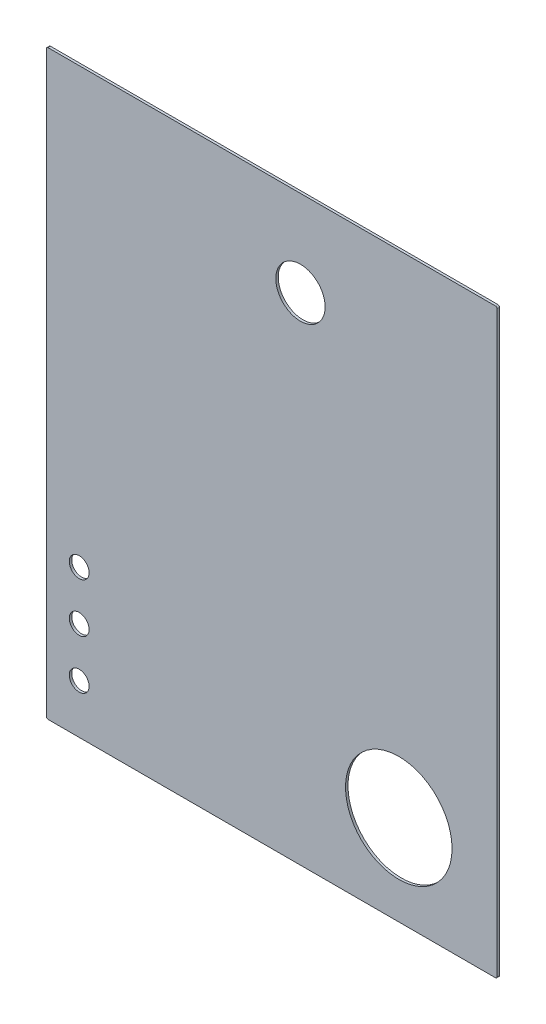
from build123d import *

# Parameters (mm, degrees)
SKETCH1_R           = 12.1
SKETCH1_R_2         = 65
SKETCH1_R_3         = 30.1
BOSS_EXTRUDE1_DEPTH = 3


with BuildPart() as part:
    # Sketch1 → Boss-Extrude1 (new body)
    with BuildSketch(Plane.XY):
        with BuildLine():
            Line((2, 0), (548, 0))
            ThreePointArc((548, 0), (549.414213562, 0.585786438), (550, 2))
            Line((550, 2), (550, 708))
            ThreePointArc((550, 708), (549.414213562, 709.414213562), (548, 710))
            Line((548, 710), (2, 710))
            ThreePointArc((2, 710), (0.585786438, 709.414213562), (0, 708))
            Line((0, 708), (0, 2))
            ThreePointArc((0, 2), (0.585786438, 0.585786438), (2, 0))
        make_face()
        with Locations((40, 60)):
            Circle(SKETCH1_R, mode=Mode.SUBTRACT)
        with Locations((40, 120)):
            Circle(SKETCH1_R, mode=Mode.SUBTRACT)
        with Locations((40, 180)):
            Circle(SKETCH1_R, mode=Mode.SUBTRACT)
        with Locations((430, 110)):
            Circle(SKETCH1_R_2, mode=Mode.SUBTRACT)
        with Locations((310, 605)):
            Circle(SKETCH1_R_3, mode=Mode.SUBTRACT)
    extrude(amount=BOSS_EXTRUDE1_DEPTH)


solid = part.part
